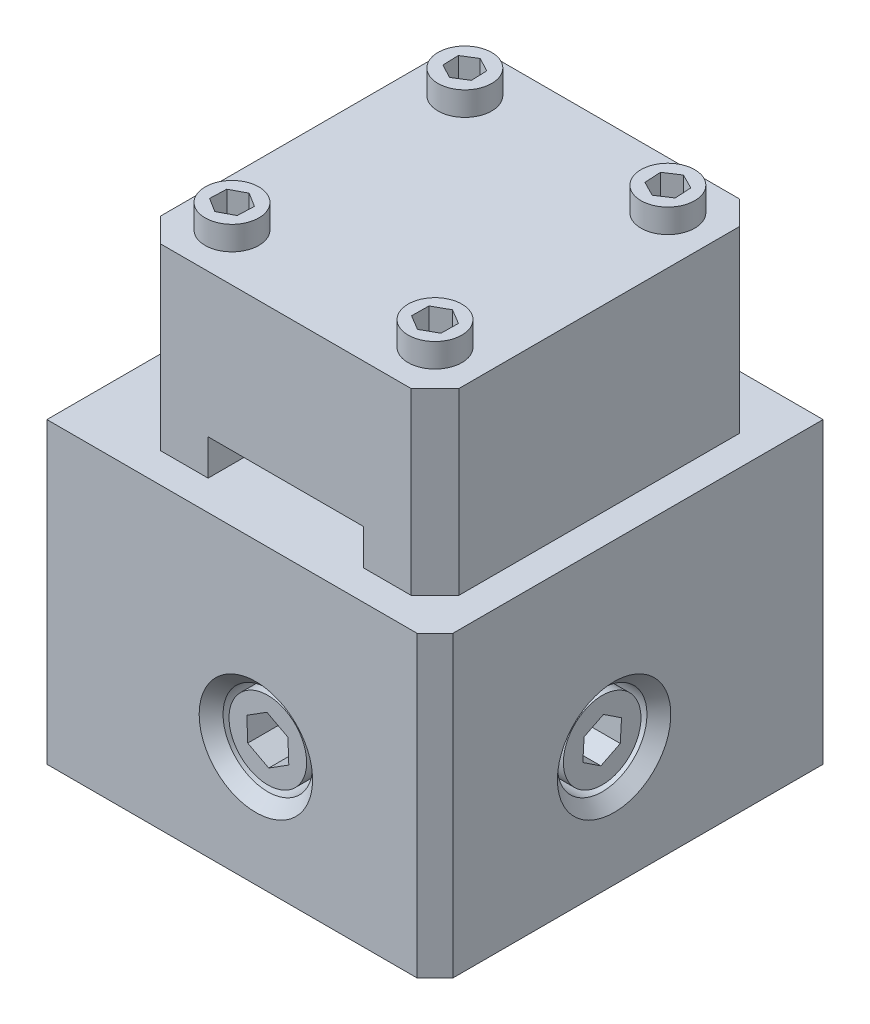
from build123d import *

# Parameters (mm, degrees)
BOSS_EXTRUDE1_DEPTH  = 40
SKETCH3_W            = 65
SKETCH3_H            = 65
BOSS_EXTRUDE3_DEPTH  = 10
SKETCH4_R            = 7.5
CUT_EXTRUDE1_DEPTH   = 10
SKETCH5_R            = 7.5
CUT_EXTRUDE2_DEPTH   = 10
SKETCH6_R            = 6.5
BOSS_EXTRUDE4_DEPTH  = 8
SKETCH7_R            = 6.5
BOSS_EXTRUDE5_DEPTH  = 8
CHAMFER1_SIZE        = 2
CHAMFER2_SIZE        = 3
BOSS_EXTRUDE6_DEPTH  = 55
SKETCH10_W           = 55
SKETCH10_H           = 30
CUT_EXTRUDE3_DEPTH   = 5
SKETCH12_W           = 40.885707084
SKETCH12_H           = 30.580268586
BOSS_EXTRUDE10_DEPTH = 5
SKETCH13_W           = 26
SKETCH13_H           = 6
CUT_EXTRUDE4_DEPTH   = 65
SKETCH14_R           = 4.5
BOSS_EXTRUDE11_DEPTH = 4
CHAMFER3_SIZE        = 4


with BuildPart() as part:
    # Sketch1 → Boss-Extrude1 (new body)
    with BuildSketch(Plane(origin=(0, 0, 0), x_dir=(1, 0, 0), z_dir=(0, 1, 0))):
        Polygon((20, 20), (20, 35), (30, 35), (30, -30), (-35, -30), (-35, -20), (-20, -20), (-20, 20), align=None)
    extrude(amount=BOSS_EXTRUDE1_DEPTH)

    # Sketch3 → Boss-Extrude3 (add)
    with BuildSketch(Plane(origin=(0, 40, 0), x_dir=(1, 0, 0), z_dir=(0, 1, 0))):
        with Locations((-2.5, 2.5)):
            Rectangle(SKETCH3_W, SKETCH3_H)
    extrude(amount=BOSS_EXTRUDE3_DEPTH)

    # Sketch4 → Cut-Extrude1 (cut)
    with BuildSketch(Plane.XY.offset(30)):
        with Locations((0, 20)):
            Circle(SKETCH4_R)
    extrude(amount=-CUT_EXTRUDE1_DEPTH, mode=Mode.SUBTRACT)

    # Sketch5 → Cut-Extrude2 (cut)
    with BuildSketch(Plane(origin=(30, 0, 0), x_dir=(0, 0, -1), z_dir=(1, 0, 0))):
        with Locations((0, 20)):
            Circle(SKETCH5_R)
    extrude(amount=-CUT_EXTRUDE2_DEPTH, mode=Mode.SUBTRACT)

    # Sketch6 → Boss-Extrude4 (add)
    with BuildSketch(Plane.XY.offset(20)):
        with Locations((0, 20)):
            Circle(SKETCH6_R)
        Polygon((3.513043884, 18.143020132), (3.364713682, 22.113895314), (-0.148330202, 23.970875182), (-3.513043884, 21.856979868), (-3.364713682, 17.886104686), (0.148330202, 16.029124818), align=None, mode=Mode.SUBTRACT)
    extrude(amount=BOSS_EXTRUDE4_DEPTH)

    # Sketch7 → Boss-Extrude5 (add)
    with BuildSketch(Plane(origin=(20, 0, 0), x_dir=(0, 0, -1), z_dir=(1, 0, 0))):
        with Locations((0, 20)):
            Circle(SKETCH7_R)
        Polygon((3.02745999, 18.002364135), (3.243733401, 21.623039328), (0.216273412, 23.620675193), (-3.02745999, 21.997635865), (-3.243733401, 18.376960672), (-0.216273412, 16.379324807), align=None, mode=Mode.SUBTRACT)
    extrude(amount=BOSS_EXTRUDE5_DEPTH)

    # Chamfer1
    chamfer1_edges = [part.edges().sort_by_distance(p)[0] for p in [
        (-7.5, 20, 30),
        (30, 20, 7.5),
    ]]
    chamfer(chamfer1_edges, length=CHAMFER1_SIZE)

    # Chamfer2
    chamfer2_edges = [part.edges().sort_by_distance(p)[0] for p in [
        (30, 25, 30),
    ]]
    chamfer(chamfer2_edges, length=CHAMFER2_SIZE)

    # Sketch9 → Boss-Extrude6 (add)
    with BuildSketch(Plane(origin=(30, 0, 0), x_dir=(0, 0, -1), z_dir=(1, 0, 0))):
        Polygon((-25, 50), (-25, 80), (30, 80), (30, 50), (20, 50), (20, 75), (-15, 75), (-15, 50), align=None)
    extrude(amount=-BOSS_EXTRUDE6_DEPTH)

    # Sketch10 → Cut-Extrude3 (cut)
    with BuildSketch(Plane(origin=(30, 0, 0), x_dir=(0, 0, -1), z_dir=(1, 0, 0))):
        with Locations((2.5, 65)):
            Rectangle(SKETCH10_W, SKETCH10_H)
    extrude(amount=-CUT_EXTRUDE3_DEPTH, mode=Mode.SUBTRACT)

    # Sketch12 → Boss-Extrude10 (add)
    with BuildSketch(Plane(origin=(25, 0, 0), x_dir=(0, 0, -1), z_dir=(1, 0, 0))):
        with Locations((2.5, 60.722892632)):
            Rectangle(SKETCH12_W, SKETCH12_H)
    extrude(amount=-BOSS_EXTRUDE10_DEPTH)

    # Sketch13 → Cut-Extrude4 (cut)
    with BuildSketch(Plane.XY.offset(25)):
        with Locations((0, 53)):
            Rectangle(SKETCH13_W, SKETCH13_H)
    extrude(amount=-CUT_EXTRUDE4_DEPTH, mode=Mode.SUBTRACT)

    # Sketch14 → Boss-Extrude11 (add)
    # profile 1 of 4: a face of its own
    with BuildSketch(Plane(origin=(0, 80, 0), x_dir=(1, 0, 0), z_dir=(0, 1, 0))):
        with Locations(Location((-17, 22, 0), (0, 0, 270))):
            Circle(SKETCH14_R)
        Polygon((-14.650196001, 20.748047177), (-14.740875051, 23.409013546), (-17.090679051, 24.660966369), (-19.349803999, 23.251952823), (-19.259124949, 20.590986454), (-16.909320949, 19.339033631), align=None, mode=Mode.SUBTRACT)
    # profile 2 of 4: a face of its own
    with BuildSketch(Plane(origin=(0, 80, 0), x_dir=(1, 0, 0), z_dir=(0, 1, 0))):
        with Locations(Location((17, 22, 0), (0, 0, 270))):
            Circle(SKETCH14_R)
        Polygon((19.479568046, 20.748047177), (19.324006972, 23.521392507), (16.844438926, 24.77334533), (14.520431954, 23.251952823), (14.675993028, 20.478607493), (17.155561074, 19.22665467), align=None, mode=Mode.SUBTRACT)
    # profile 3 of 4: a face of its own
    with BuildSketch(Plane(origin=(0, 80, 0), x_dir=(1, 0, 0), z_dir=(0, 1, 0))):
        with Locations(Location((17, -17, 0), (0, 0, 270))):
            Circle(SKETCH14_R)
        Polygon((19.479568046, -18.478428301), (19.520140489, -15.591845232), (17.040572443, -14.113416931), (14.520431954, -15.521571699), (14.479859511, -18.408154768), (16.959427557, -19.886583069), align=None, mode=Mode.SUBTRACT)
    # profile 4 of 4: a face of its own
    with BuildSketch(Plane(origin=(0, 80, 0), x_dir=(1, 0, 0), z_dir=(0, 1, 0))):
        with Locations(Location((-17, -17, 0), (0, 0, 270))):
            Circle(SKETCH14_R)
        Polygon((-14.650196001, -18.478428301), (-14.544741534, -15.704224193), (-16.894545533, -14.225795892), (-19.349803999, -15.521571699), (-19.455258466, -18.295775807), (-17.105454467, -19.774204108), align=None, mode=Mode.SUBTRACT)
    extrude(amount=BOSS_EXTRUDE11_DEPTH)

    # Chamfer3
    chamfer3_edges = [part.edges().sort_by_distance(p)[0] for p in [
        (-25, 65, 25),
        (-25, 65, -30),
        (25, 65, 25),
        (25, 65, -30),
    ]]
    chamfer(chamfer3_edges, length=CHAMFER3_SIZE)


solid = part.part
